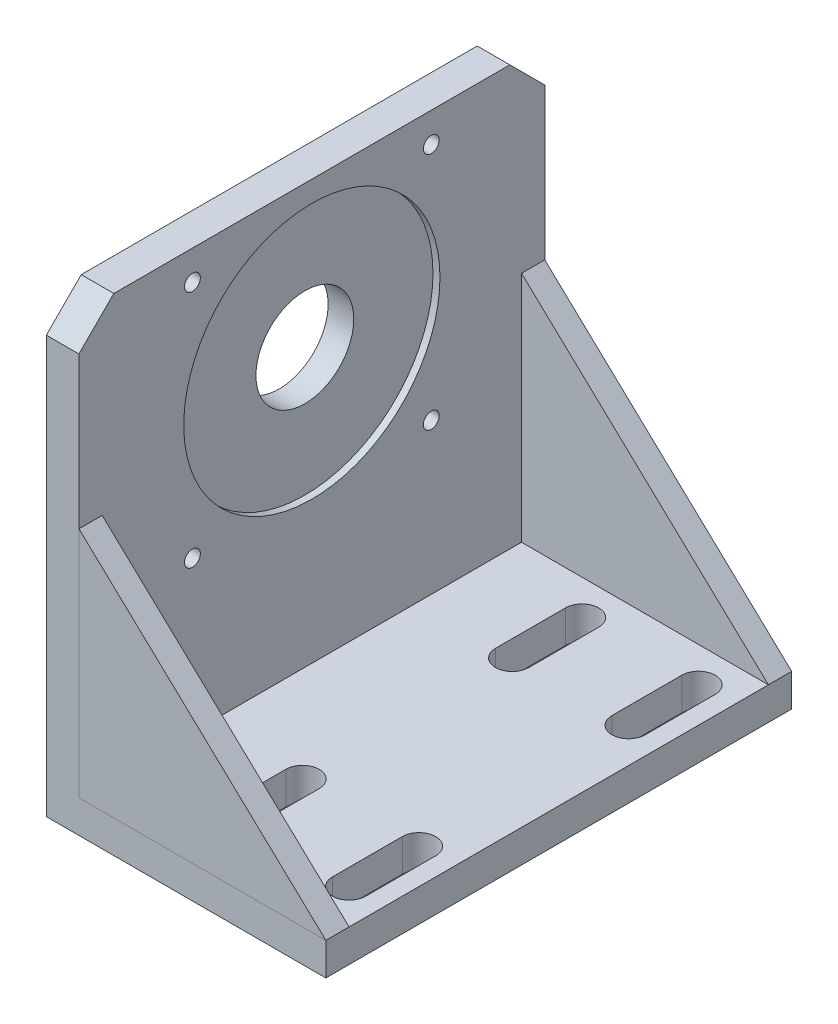
SolidWorks part; units mm, degrees
ref_plane "前视基准面" through (0, 0, 0) normal (0, 0, 1) x (1, 0, 0)
ref_plane "上视基准面" through (0, 0, 0) normal (0, 1, 0) x (1, 0, 0)
ref_plane "右视基准面" through (0, 0, 0) normal (1, 0, 0) x (0, 0, -1)
sketch "草图1" plane through (0, 0, 0) normal (0, 1, 0) x (1, 0, 0)
  line L1 (-60, 100) -> (60, 100)
  line L2 (-60, 100) -> (-60, -100)
  line L3 (-60, -100) -> (60, -100)
  line L4 (60, 100) -> (60, -100)
  line L5 (-60, 100) -> (60, -100) construction
  line L6 (-60, -100) -> (60, 100) construction
  point P0 (0, 0)
  dimension "D1" = 120
  dimension "D2" = 200
extrude "凸台-拉伸1" add sketch "草图1" along normal blind 14
sketch "草图2" plane through (0, 14, 0) normal (0, 1, 0) x (1, 0, 0)
  line L0 (-60, -100) -> (60, -100) construction
  line L1 (-60, 100) -> (-46, 100)
  line L2 (-60, 100) -> (-60, -100)
  line L3 (-60, -100) -> (-46, -100)
  line L4 (-46, 100) -> (-46, -100)
  dimension "D1" = 14
extrude "凸台-拉伸2" add sketch "草图2" along normal blind 180
sketch "草图3" plane through (0, 0, 100) normal (0, 0, 1) x (1, 0, 0)
  line L0 (-46, 114) -> (60, 14)
  line L1 (-46, 194) -> (-46, 14) construction
  line L2 (-46, 14) -> (60, 14) construction
  line L3 (-46, 114) -> (-46, 14)
  line L4 (-46, 14) -> (60, 14)
  dimension "D1" = 100
extrude "凸台-拉伸3" add sketch "草图3" against normal blind 10 separate body
sketch "草图4" plane through (0, 0, -100) normal (0, 0, -1) x (-1, 0, 0)
  line L3 (46, 14) -> (46, 114)
  line L4 (46, 114) -> (-60, 14)
  line L5 (46, 14) -> (46, 114)
  line L7 (46, 114) -> (-60, 14)
  line L9 (-60, 14) -> (46, 14)
  line L10 (-60, 14) -> (46, 14)
  dimension "D1" = 0
extrude "凸台-拉伸4" add sketch "草图4" against normal blind 10 separate body
sketch "草图5" plane through (-60, 0, 0) normal (-1, 0, 0) x (0, 0, 1)
  line L0 (-100, 0) -> (100, 0) construction
  circle A0 centre (0, 130) radius 21
  dimension "D1" = 130
  dimension "D2" = 42
extrude "切除-拉伸1" cut sketch "草图5" against normal blind 12
sketch "草图6" plane through (-48, 0, 0) normal (-1, 0, 0) x (0, 0, 1)
  circle A0 centre (0, 130) radius 15
  dimension "D1" = 30
extrude "切除-拉伸2" cut sketch "草图6" against normal through all
sketch "草图7" plane through (-46, 0, 0) normal (1, 0, 0) x (0, 0, -1)
  circle A0 centre (0, 130) radius 55
  dimension "D1" = 110
extrude "切除-拉伸3" cut sketch "草图7" against normal blind 3
sketch "草图8" plane through (0, 14, 0) normal (0, 1, 0) x (1, 0, 0)
  line L0 (-5, 75) -> (-5, 45) construction
  line L1 (2.1661, 75) -> (2.1661, 45)
  line L2 (-12.1661, 75) -> (-12.1661, 45)
  line L3 (45, 75) -> (45, 45) construction
  line L4 (52.1661, 75) -> (52.1661, 45)
  line L5 (37.8339, 75) -> (37.8339, 45)
  line L6 (0, 0) -> (82.4257, 0) construction
  line L7 (60, -100) -> (60, 100) construction
  line L8 (-5, -75) -> (-5, -45) construction
  line L9 (2.1661, -75) -> (2.1661, -45)
  line L10 (-12.1661, -75) -> (-12.1661, -45)
  line L11 (45, -75) -> (45, -45) construction
  line L12 (52.1661, -75) -> (52.1661, -45)
  line L13 (37.8339, -75) -> (37.8339, -45)
  arc A0 (2.1661, 75) -> (-12.1661, 75) centre (-5, 75) ccw
  arc A1 (-12.1661, 45) -> (2.1661, 45) centre (-5, 45) ccw
  arc A2 (52.1661, 75) -> (37.8339, 75) centre (45, 75) ccw
  arc A3 (37.8339, 45) -> (52.1661, 45) centre (45, 45) ccw
  arc A4 (2.1661, -75) -> (-12.1661, -75) centre (-5, -75) cw
  arc A5 (-12.1661, -45) -> (2.1661, -45) centre (-5, -45) cw
  arc A6 (52.1661, -75) -> (37.8339, -75) centre (45, -75) cw
  arc A7 (37.8339, -45) -> (52.1661, -45) centre (45, -45) cw
  point P2 (-5, 60)
  point P9 (45, 60)
  point P21 (-5, -60)
  point P28 (45, -60)
  dimension "D1" = 30
  dimension "D2" = 15
  dimension "D3" = 50
  dimension "D4" = 60
extrude "切除-拉伸4" cut sketch "草图8" against normal through all
hole_wizard "M8 螺纹孔1" positions "草图9" profile "草图10" tap size "M8" standard "GB" end condition through all
sketch "草图9" plane through (-46, 0, 0) normal (1, 0, 0) x (0, 0, -1)
  line L0 (-51.2652, 181.2652) -> (0, 130) construction
  line L1 (0, 130) -> (0, 218.0169) construction
  point P0 (-51.2652, 181.2652)
  dimension "D1" = 45
  dimension "D2" = 72.5
sketch "草图10" plane through (-46, 181.2652, 51.2652) normal (0, 1, 0) x (0, 0, -1)
  line L0 (0, 0) -> (0, 14)
  line L1 (0, 14) -> (3.4, 14)
  line L2 (3.4, 14) -> (3.4, 0)
  line L5 (3.4, 0) -> (0, 0)
  line L11 (0, -6.35) -> (0, 107.95) construction
  dimension "通孔螺纹孔钻头直径" = 6.8
  dimension "通孔螺纹孔钻头深度" = 14
cosmetic thread "孔螺蚊线1" parameters "D2"=8
pattern_circular "阵列(圆周)1" count 4 over 360 about axis through (0, 130, 0) along (1, 0, 0) of "M8 螺纹孔1"
chamfer "倒角1" distance 15 angle 45 2 edges at (-53, 194, -100) (-53, 194, 100)
